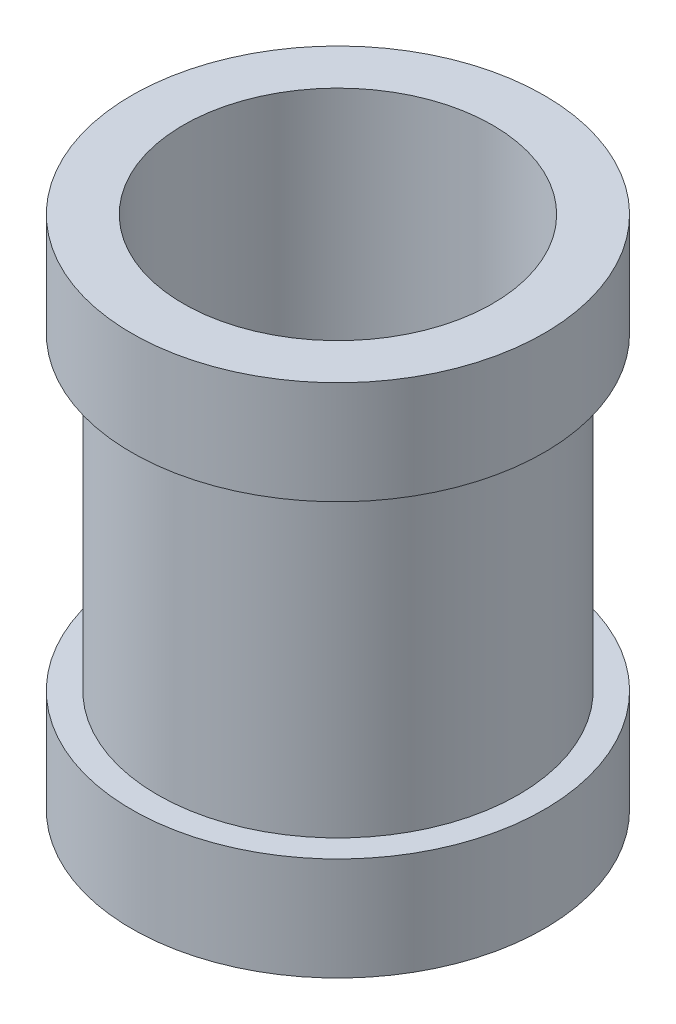
from build123d import *


with BuildPart() as part:
    # Sketch1 → Revolve1 (revolve)
    with BuildSketch(Plane.XY, mode=Mode.PRIVATE) as revolve1_sk:
        Polygon((1.5, 0), (2, 0), (2, 1), (1.75, 1), (1.75, 4), (2, 4), (2, 5), (1.5, 5), align=None)
    revolve(revolve1_sk.sketch.rotate(Axis((0, 0, 0), (0, 1, 0)), 90), axis=Axis((0, 0, 0), (0, 1, 0)))


solid = part.part
